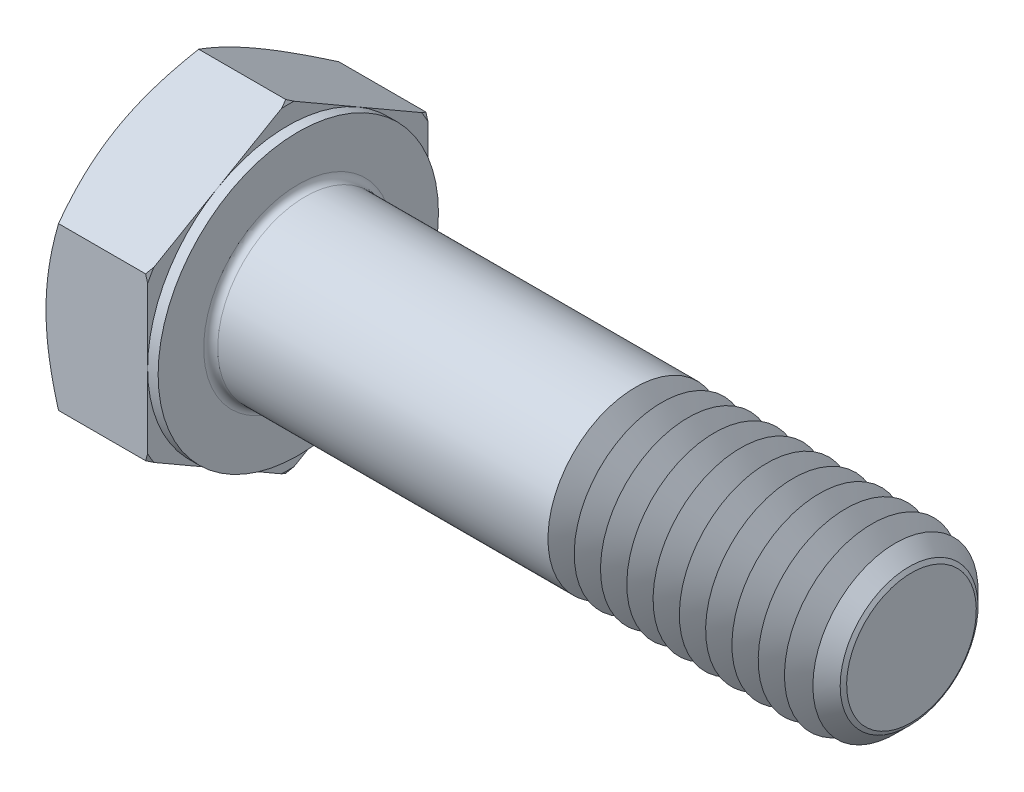
SolidWorks part; units mm, degrees
extrude "基体-拉伸" add sketch "草图1" along normal blind 6.4
sketch "草图1" plane through (0, 0, 0) normal (1, 0, 0) x (0, 0, -1)
  line L0 (8, 4.6188) -> (8, -4.6188)
  line L1 (-8, 4.6188) -> (-8, -4.6188)
  line L2 (8, -4.6188) -> (0, -9.2376)
  line L3 (0, -9.2376) -> (-8, -4.6188)
  line L4 (8, 4.6188) -> (0, 9.2376)
  line L5 (0, 9.2376) -> (-8, 4.6188)
revolve "切除-旋转1" cut sketch "草图3" angle 360 about L6
sketch "草图3" plane through (0, 0, 0) normal (0, 0, 1) x (1, 0, 0)
  line L0 (0, 8) -> (3.6013, 14.2376)
  line L1 (0, 9.2376) -> (0, 4.6188) construction
  line L2 (3.6013, 14.2376) -> (3.6013, 19.2376)
  line L3 (3.6013, 19.2376) -> (-10, 19.2376)
  line L4 (-10, 19.2376) -> (-10, 8)
  line L5 (-10, 8) -> (0, 8)
  line L6 (0, 0) -> (99.06, 0) construction
  line L7 (6.4, 9.2376) -> (0, 9.2376) construction
material "5.6级"
ref_plane "前视" through (0, 0, 0) normal (0, 0, 1) x (1, 0, 0)
ref_plane "上视" through (0, 0, 0) normal (0, 1, 0) x (1, 0, 0)
ref_plane "右视" through (0, 0, 0) normal (1, 0, 0) x (0, 0, -1)
sketch "草图2" plane through (0, 0, 0) normal (0, 0, 1) x (1, 0, 0)
  line L0 (0, 4.6188) -> (0, -4.6188) construction
  line L1 (0, 0) -> (41.4, 0)
  line L2 (0, 0) -> (0, 5)
  line L3 (0, 5) -> (7.7917, 5)
  line L4 (41.4, 0) -> (41.4, 3.701)
  line L5 (6.4, 9.2376) -> (6.4, 4.6188) construction
  line L7 (0, 0) -> (96.52, 0) construction
  line L8 (41.4, -3.701) -> (7.7917, -5) construction
  line L9 (0, -5) -> (7.7917, -5) construction
  line L10 (7.9, 15.24) -> (7.9, -1.27) construction
  line L11 (26.4, 15.24) -> (26.4, -1.27) construction
  line L12 (6.4, 4.6188) -> (6.4, -4.6188) construction
  line L13 (7.7917, 5) -> (41.4, 5)
  line L14 (41.4, 5) -> (41.4, 3.701)
revolve "凸台-旋转1" add sketch "草图2" angle 360 about L7
cosmetic thread "螺旋线1" parameters "Thread_length"=15, "Thread_minor"=7.402
sketch "草图5" plane through (0, 0, 0) normal (0, 0, 1) x (1, 0, 0)
  line L0 (6.4, 8) -> (2.7987, 14.2376)
  line L1 (6.4, 9.2376) -> (6.4, 4.6188) construction
  line L2 (2.7987, 14.2376) -> (2.7987, 19.2376)
  line L3 (2.7987, 19.2376) -> (12.7987, 19.2376)
  line L4 (12.7987, 19.2376) -> (12.7987, 8)
  line L5 (12.7987, 8) -> (6.4, 8)
  line L7 (6.4, 9.2376) -> (0.7145, 9.2376) construction
  line L8 (0, 0) -> (99.06, 0) construction
  line L9 (0, 0) -> (99.06, 0) construction
revolve "切除-旋转2" cut sketch "草图5" angle 360 about L8
sketch "草图4" plane through (0, 0, 0) normal (0, 0, 1) x (1, 0, 0)
  line L1 (6.4, 9.2376) -> (6.4, 4.6188) construction
  line L2 (6.4, 8) -> (5.8, 8)
  line L3 (6.4, 8) -> (6.4, 19.2376)
  line L4 (6.4, 19.2376) -> (5.8, 19.2376)
  line L5 (0, 0) -> (95.25, 0) construction
  line L6 (0, 0) -> (96.52, 0) construction
  line L7 (5.8, 8) -> (5.8, 19.2376)
  line L8 (5.6855, 9.2376) -> (0.7145, 9.2376) construction
revolve "切除-旋转3" cut sketch "草图4" angle 360 about L5
chamfer "倒角" distance 1.2 angle 45 1 edges at (41.4, 0, 5)
fillet "圆角" radius 0.4 1 edges at (6.4, 0, -5)
sketch "草图6" plane through (0, 0, 0) normal (0, 0, 1) x (1, 0, 0)
  line L0 (26.4, -3.701) -> (25.65, -5)
  line L1 (26.4, -3.701) -> (27.15, -5)
  line L2 (27.15, -5) -> (27.15, -6.25)
  line L3 (-3.175, 0) -> (5.1513, 0) construction
  line L5 (27.15, -6.25) -> (25.65, -6.25)
  line L6 (25.65, -6.25) -> (25.65, -5)
revolve "切除-旋转4" cut sketch "草图6" angle 360 about L3
pattern_linear "阵列(线性)1" count 11 spacing 1.5 along (1, 0, 0) of "切除-旋转4"
equation "\"D3@草图1\" = \"s@草图1\" / 2"
equation "\"D4@草图1\" = \"D3@草图1\""
equation "\"D5@草图1\" = \"D4@草图1\""
equation "\"Thread_minor@螺旋线1\" = \"Minor_dia@草图2\""
equation "\"D1@草图3\" = \"s@草图1\" / 2"
equation "\"D1@草图5\" = \"s@草图1\" / 2"
equation "\"Head_ch_ang@草图5\" = \"Head_ch_ang@草图3\""
equation "\"D1@草图4\" = \"s@草图1\""
equation "\"Thread_length@螺旋线1\" = ((sgn( (\"l@草图2\" - \"p@草图2\" ) - \"h@草图2\" )-1)*( (\"l@草图2\" - \"p@草图2\" ) - \"h@草图2\" ))/-2+ \"h@草图2\""
equation "\"Thread_minor@草图6\" = \"Minor_dia@草图2\""
equation "\"Diameter@草图6\" = \"m@草图2\""
equation "\"Overcut@草图6\" = \"m@草图2\" * 1.25"
equation "\"Start@草图6\" = \"k@基体-拉伸\" + \"l@草图2\" - \"Thread_length@螺旋线1\"  '---Non-countersunk---"
equation "\"Num_threads@阵列(线性)1\" = int( \"Thread_length@螺旋线1\" / \"p@草图2\" + 0.999 )  + 1"
equation "\"Advance@阵列(线性)1\" = \"Thread_length@螺旋线1\" /  (\"Num_threads@阵列(线性)1\" - 1) 'relax it"
equation "\"Num_threads@阵列(线性)1\" = \"Num_threads@阵列(线性)1\" - sgn( \"Num_threads@阵列(线性)1\" - 1) '---chamfered tips only---"
equation "\"Minor_dia@草图2\" = \"m@草图2\"-\"p@草图2\" * 1.732"
equation "\"D1@倒角\" = \"p@草图2\"*0.8"
